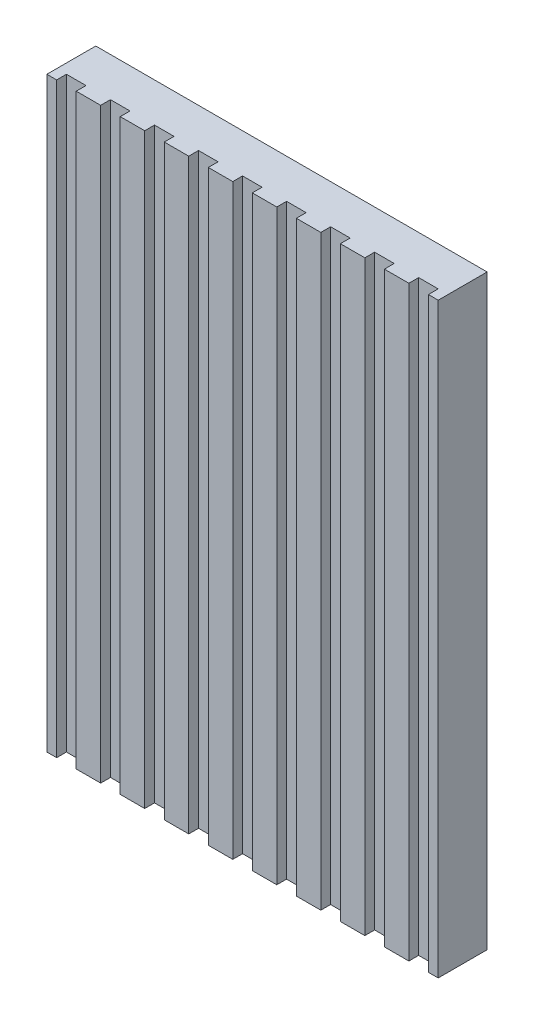
from build123d import *

# Parameters (mm, degrees)
SKETCH1_W           = 800
SKETCH1_H           = 1200
BOSS_EXTRUDE1_DEPTH = 100
SKETCH2_W           = 40
SKETCH2_H           = 40
CUT_EXTRUDE1_DEPTH  = 1269.857754045
LPATTERN1_COUNT     = 5
LPATTERN1_PITCH     = 90
LPATTERN1_COL_COUNT = 5
LPATTERN1_COL_PITCH = 90


with BuildPart() as part:
    # Sketch1 → Boss-Extrude1 (new body)
    with BuildSketch(Plane.XY):
        Rectangle(SKETCH1_W, SKETCH1_H)
    extrude(amount=BOSS_EXTRUDE1_DEPTH)

    # Sketch2 → Cut-Extrude1 (cut, through all)
    with BuildSketch(Plane.XZ.offset(600)):
        with Locations((0, 100)):
            Rectangle(SKETCH2_W, SKETCH2_H)
    cut_extrude1 = extrude(amount=-CUT_EXTRUDE1_DEPTH, mode=Mode.SUBTRACT)

    # LPattern1: Cut-Extrude1 ×5
    with Locations(*[(i * LPATTERN1_PITCH, 0, 0) for i in range(1, LPATTERN1_COUNT)]):
        add(cut_extrude1, mode=Mode.SUBTRACT)

    # LPattern1 col: Cut-Extrude1 ×5
    with Locations(*[(-i * LPATTERN1_COL_PITCH, 0, 0) for i in range(1, LPATTERN1_COL_COUNT)]):
        add(cut_extrude1, mode=Mode.SUBTRACT)


solid = part.part
